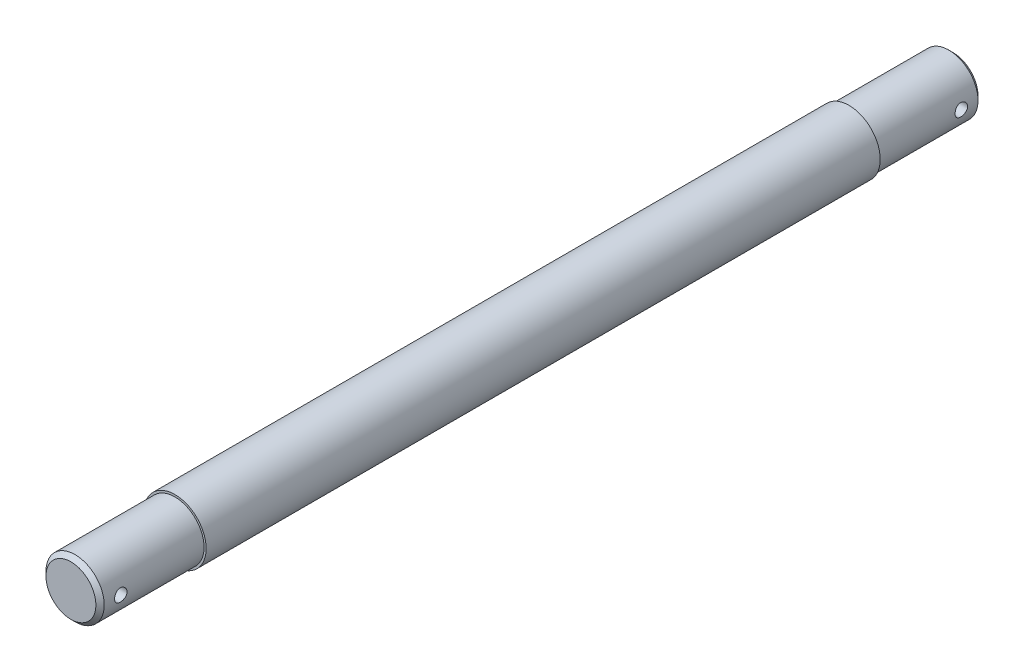
SolidWorks part; units mm, degrees
material "Q235B"
ref_plane "Front Plane" through (0, 0, 0) normal (0, 0, 1) x (1, 0, 0)
ref_plane "Top Plane" through (0, 0, 0) normal (0, 1, 0) x (1, 0, 0)
ref_plane "Right Plane" through (0, 0, 0) normal (1, 0, 0) x (0, 0, -1)
other "Configuration Table"
sketch "Sketch1" plane through (0, 0, 0) normal (1, 0, 0) x (0, 0, -1)
  line L1 (0, 0) -> (25, 0)
  line L2 (0, 0) -> (0, 7)
  line L3 (0, 7) -> (25, 7)
  line L4 (25, 0) -> (25, 7)
  line L5 (25, 0) -> (187, 0)
  line L6 (25, 0) -> (25, 7.5)
  line L7 (25, 7.5) -> (187, 7.5)
  line L8 (187, 0) -> (187, 7.5)
  line L9 (187, 0) -> (212, 0)
  line L10 (187, 0) -> (187, 7)
  line L11 (187, 7) -> (212, 7)
  line L12 (212, 0) -> (212, 7)
  dimension "D1" = 7
  dimension "D2" = 7
  dimension "D3" = 162
  dimension "D4" = 212
  dimension "D5" = 25
  dimension "D6" = 7.5
revolve "Revolve1" add sketch "Sketch1" angle 360 about L5
sketch "Sketch2" plane through (0, 0, 0) normal (1, 0, 0) x (0, 0, -1)
  line L0 (187, -7) -> (187, 7) construction
  line L1 (25, 7) -> (25, -7) construction
  circle A0 centre (5, 0) radius 1.5
  circle A1 centre (207, 0) radius 1.5
  dimension "D1" = 3
  dimension "D2" = 20
  dimension "D3" = 20
  dimension "D4" = 0
  dimension "D5" = 0
extrude "Cut-Extrude1" cut sketch "Sketch2" against normal through all both and the other way through all
chamfer "Chamfer1" distance 1 angle 45 2 edges at (7, 0, -212) (7, 0, 0)
